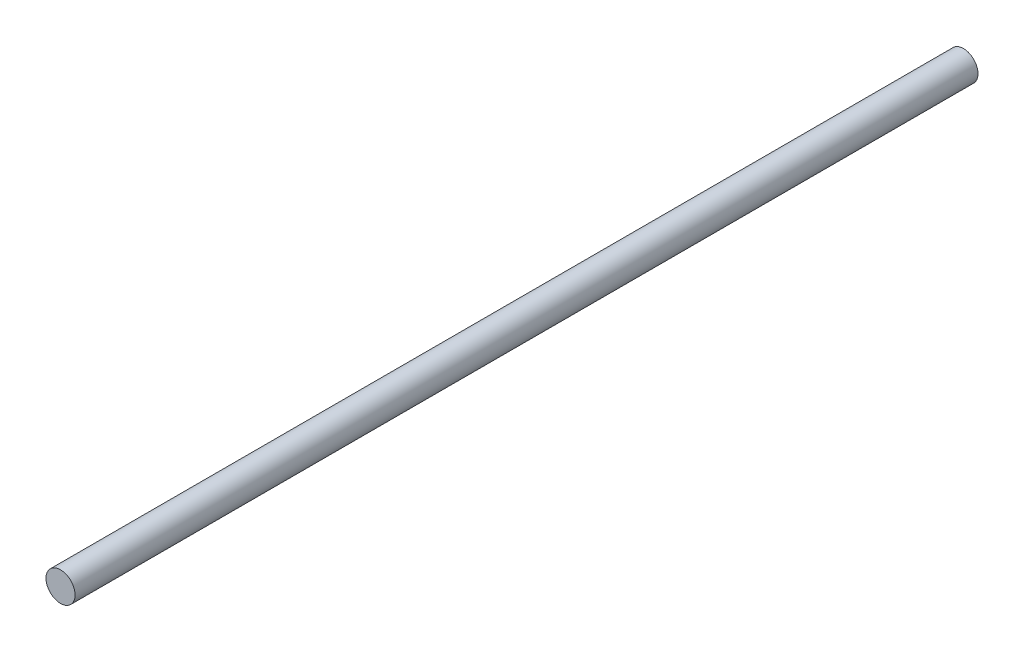
from build123d import *

# Parameters (mm, degrees)
SKETCH1_R           = 2
BOSS_EXTRUDE1_DEPTH = 62


with BuildPart() as part:
    # Sketch1 → Boss-Extrude1 (new, symmetric)
    with BuildSketch(Plane.XY):
        Circle(SKETCH1_R)
    extrude(amount=BOSS_EXTRUDE1_DEPTH, both=True)


solid = part.part
